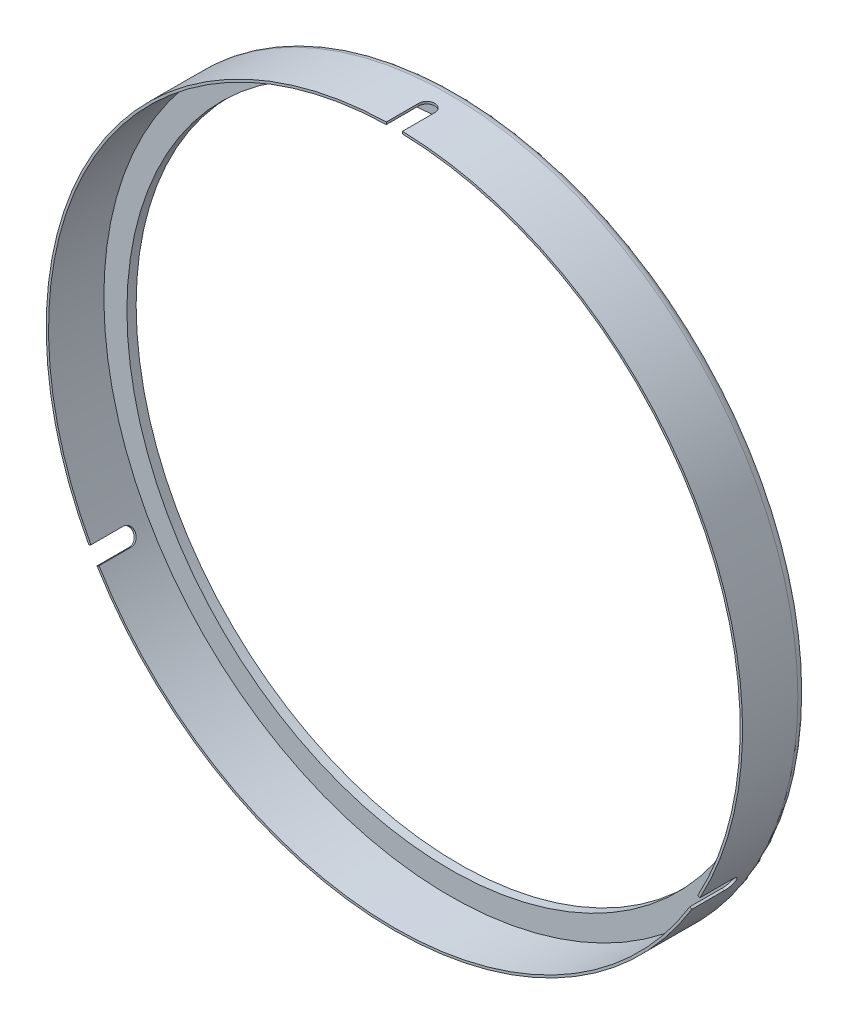
SolidWorks part; units mm, degrees
ref_plane "Front plane" through (0, 0, 0) normal (0, 0, 1) x (1, 0, 0)
ref_plane "Top plane" through (0, 0, 0) normal (0, 1, 0) x (1, 0, 0)
ref_plane "Right plane" through (0, 0, 0) normal (1, 0, 0) x (0, 0, -1)
sketch "Sketch 1" plane through (0, 0, 0) normal (0, 0, 1) x (1, 0, 0)
  circle A0 centre (0, 0) radius 75.5
  circle A1 centre (0, 0) radius 71
  circle A2 centre (0, 0) radius 75
  dimension "D1" = 151
  dimension "D2" = 142
  dimension "D3" = 150
extrude "Boss-Extrude 1" add sketch "Sketch 1" along normal blind 14 contours A2 | A0
sketch "Sketch 2" plane through (0, 0, 0) normal (0, 0, 1) x (1, 0, 0)
  circle A2 centre (0, 0) radius 75 construction
  circle A3 centre (0, 0) radius 75
extrude "Boss-Extrude 2" add sketch "Sketch 2" along normal blind 2
sketch "Sketch 3" plane through (0, 0, 0) normal (0, 0, -1) x (-1, 0, 0)
  circle A0 centre (0, 0) radius 70
  dimension "D1" = 140
extrude "Cut-Extrude 1" cut sketch "Sketch 3" against normal up to next
ref_plane "Reference plane 1" through (0, 75.5, 0) normal (0, 1, 0) x (1, 0, 0)
sketch "Sketch 7" plane through (0, 75.5, 0) normal (0, 1, 0) x (1, 0, 0)
  line L0 (0, 0) -> (0, -14)
  line L1 (-75.5, -14) -> (75.5, -14) construction
  line L2 (0, -14) -> (1.75, -14)
  line L3 (1.75, -14) -> (1.75, -7)
  line L4 (0, -14) -> (-1.75, -14)
  line L5 (-1.75, -14) -> (-1.75, -7)
  arc A0 (-1.75, -7) -> (1.75, -7) centre (0, -7) cw
  dimension "D1" = 1.75
  dimension "D2" = 1.75
  dimension "D3" = 7
  dimension "D4" = 7
extrude "Cut-Extrude 3" cut sketch "Sketch 7" against normal up to next contours A0 L5 L4 L0 | A0 L0 L2 L3
pattern_circular "Circular pattern 1" count 3 over 360 about axis through (0, 0, 0) along (0, 0, 1) of "Cut-Extrude 3"
fillet "Fillet 1" radius 2 1 edges at (75.5, 0, 0)
